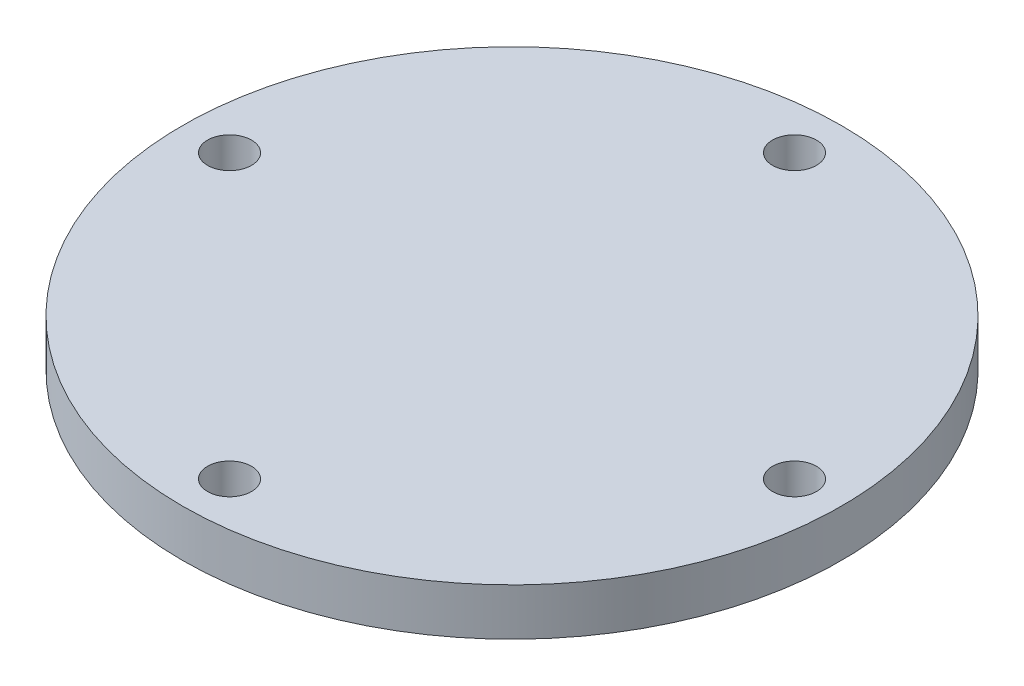
from build123d import *

# Parameters (mm, degrees)
SKETCH1_R                  = 105
BOSS_EXTRUDE1_DEPTH        = 15
F_14_0_14_DIAMETER_HOLE1_D = 14


with BuildPart() as part:
    # Sketch1 → Boss-Extrude1 (new body)
    with BuildSketch(Plane(origin=(0, 0, 0), x_dir=(1, 0, 0), z_dir=(0, 1, 0))):
        with Locations(Location((0, 0, 0), (0, 0, 270))):
            Circle(SKETCH1_R)
    extrude(amount=BOSS_EXTRUDE1_DEPTH)

    # Ø14.0 (14) Diameter Hole1 (through all)
    with Locations(Plane(origin=(0, 15, 0), x_dir=(1, 0, 0), z_dir=(0, 1, 0))):
        with Locations((0, 90), (90, 0), (0, -90), (-90, 0)):
            Hole(F_14_0_14_DIAMETER_HOLE1_D / 2)


solid = part.part
